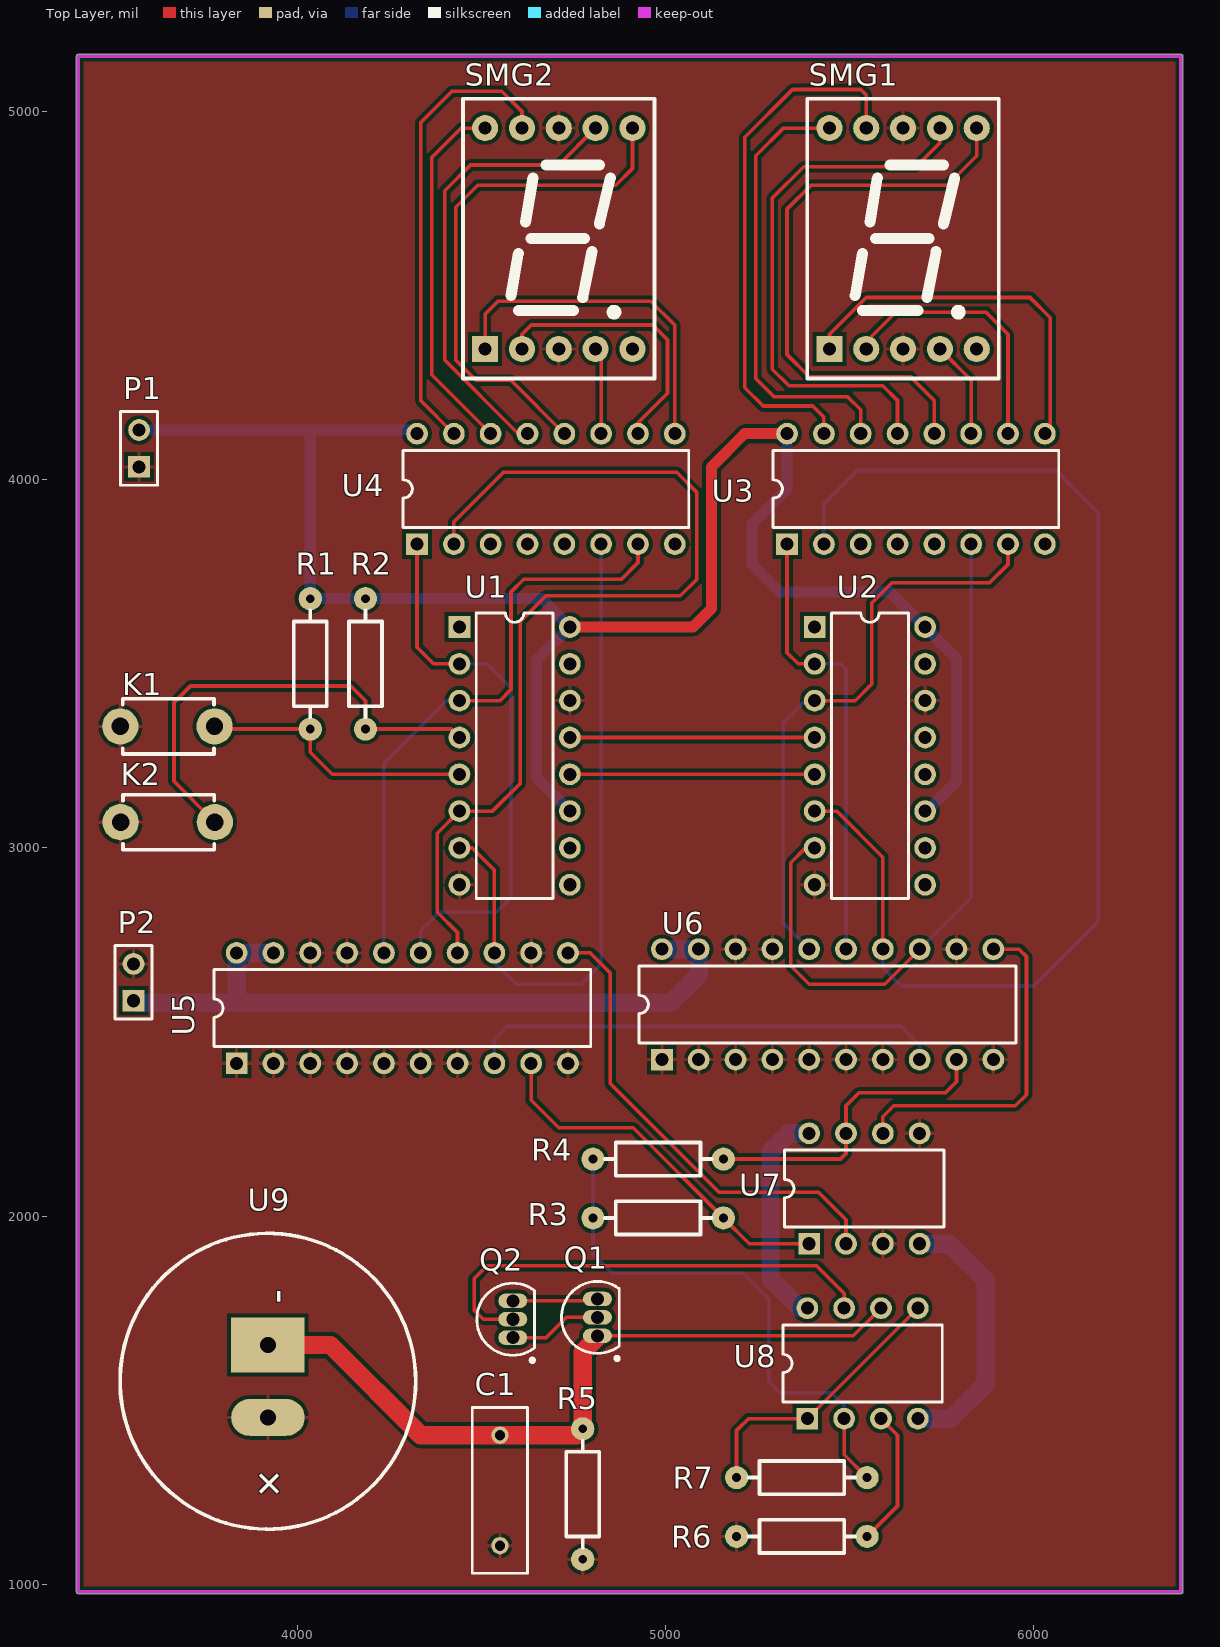
[diagram p0: Top Layer view]
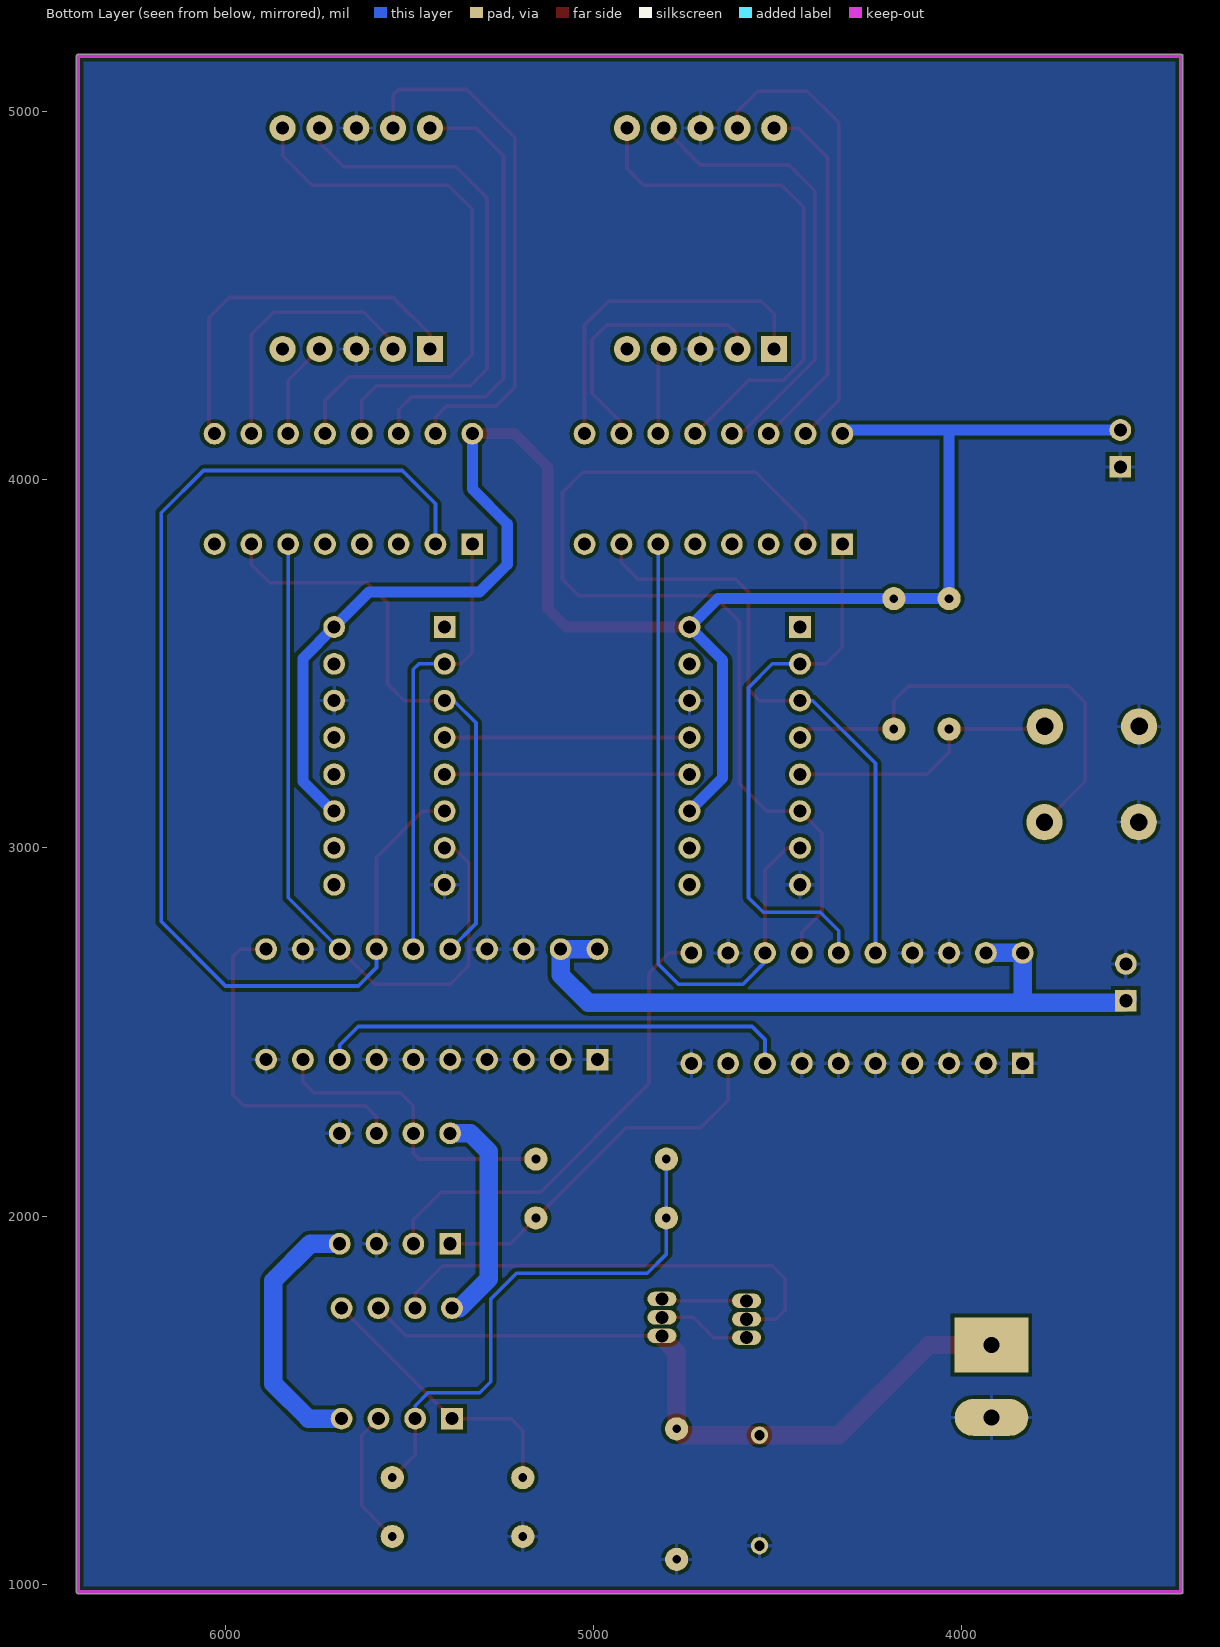
[diagram p1: Bottom Layer view, seen from below]
# Altium PCB MISC84311.PcbDoc
Units mil, origin at the board's own origin, x right, y up, seen from the top; angles counter-clockwise.
Board outline 3005.03 x 4180.03 mil, 2 copper layers (Top Layer, Bottom Layer); 25 components, 43 nets, 172 pads, 0 vias.

## Layer stack, top to bottom (the 12.6 mil dielectric is the usual default, probably not edited)
Top Solder: solder mask 0.4, Solder Resist, Dk 3.5
Top Layer: signal copper 1.4
Dielectric 1: dielectric 12.6, FR-4, Dk 4.8
Bottom Layer: signal copper 1.4
Bottom Solder: solder mask 0.4, Solder Resist, Dk 3.5

## Board outline
3399.99,980 ccw(c3405,980) 3405,974.99 6400,974.99 ccw(c6400,980) 6405.02,980 6405.02,5150 ccw(c6400,5150) 6400,5155.02 3405,5155.02 ccw(c3405,5150) 3399.99,5150

## Design rules (kind name [scope] priority, off if disabled: settings)
Clearance [All] p1: gap=10
HoleSize [All] p1: absolutevalues=TRUE maxlimit=99999 minlimit=1 maxpercent=80.000 minpercent=20.000
MinimumSolderMaskSliver [All] p1: minsoldermaskwidth=0
PolygonConnect [All] p1: connectstyle=Relief reliefconductorwidth=10 reliefentries=4 polygonreliefangle="90 Angle" airgapwidth=10
RoutingVias [All] p1: holewidth=28 width=50 viastyle="Through Hole" minholewidth=28 minwidth=50 maxholewidth=28 maxwidth=50
SilkToSilkClearance [All] p1: silktosilkclearance=0
SilkToSolderMaskClearance [IsPad] p1: minsilkscreentomaskgap=0 clearancetoexposedcopper=TRUE
SolderMaskExpansion [All] p1: expansion=4
Width [All] p1: maxlimit=50 minlimit=10 preferedwidth=10
26 further rules are at their usual default settings.

## Components (designator, comment, footprint, x,y, rotation, side; value= is the part's Value field where it differs from the comment)
C1 "100UF" RAD-0.3 4550,1255 r90 top
K1 "KEY" DIP-3X6X4.3 3519.09,3330 r0 top
K2 "KEY" DIP-3X6X4.3 3520,3070 r0 top
P1 "Header 2" HDR1X2 3570,4035 r90 top
P2 "Header 2" HDR1X2 3555,2585 r90 top
Q1 "2N3055" TO-92A 4815,1725 r0 top
Q2 "2N3904" TO-92A 4585,1720 r0 top
R1 "10K" "RS 1/4W" 4035,3500 r90 top
R2 "10K" "RS 1/4W" 4185,3500 r90 top
R3 "100K" "RS 1/4W" 4980,1995 r0 top
R4 "10K" "RS 1/4W" 4980,2155 r0 top
R5 "10K" "RS 1/4W" 4775,1245 r270 top
R6 "10K" "RS 1/4W" 5370,1130 r0 top
R7 "10K" "RS 1/4W" 5370,1290 r180 top
SMG1 "5011A" "SMG 0.5-1P" 5645,4655 r0 top
SMG2 "5011A" "SMG 0.5-1P" 4710,4655 r0 top
U1 "SN74LS192N" 648-08 4590,3250 r270 top
U2 "SN74LS192N" 648-08 5555,3250 r270 top
U3 "SN74LS48N" N016D 5680,3975 r0 top
U4 "SN74LS48N" N016D 4675,3975 r0 top
U5 "DAC0832" J20A 4285,2565 r0 top
U6 "DAC0832" J20A 5440,2575 r0 top
U7 "NE5532" P008 5540,2075 r0 top
U8 "NE5532" P008 5535,1600 r0 top
U9 "Volts" "CAPACITANCE 1 FARAD 5,5 VOLT" 3920,1551.58 r90 top

## Footprints (in the part's own frame and the unit in brackets; to place one, negate y for a bottom-side part, rotate by r counter-clockwise, add the part's x,y. Pads: shape width x height; smd on the part's side, far side on the other; paste and mask are expansions set on the pad)
648-08 [mm] "DIP; 16 Leads; Row Spacing 7.62 mm; Pitch 2.54 mm"
  rect 1.5x1.5 hole 0.9: 1(-8.89,-3.81)
  round 1.5 hole 0.9: 2(-6.35,-3.81) 3(-3.81,-3.81) 4(-1.27,-3.81) 5(1.27,-3.81) 6(3.81,-3.81) 7(6.35,-3.81) 8(8.89,-3.81) 9(8.89,3.81) 10(6.35,3.81) 11(3.81,3.81) 12(1.27,3.81) 13(-1.27,3.81) 14(-3.81,3.81) 15(-6.35,3.81) 16(-8.89,3.81)
  silkscreen extent -9.85,-2.65 9.85,2.65
"CAPACITANCE 1 FARAD 5,5 VOLT" [mil]
  rect 150x200 hole 43.31 paste+0 mask+2: 1(98.42,0)
  oval 100x200 hole 43.31 paste+0 mask+2: 2(-98.4,0)
  silkscreen extent -402,-402 402,401
DIP-3X6X4.3 [mm]
  round 2.5 hole 1.2: 1(0,0) 3(6.5,0)
  silkscreen extent 0.16,-1.9 6.46,1.9, body extent -0.64,-1.75 7.19,1.75, height 4.31
HDR1X2 [mm] "Connector; Header; 2 Position"
  rect 1.5x1.5 hole 0.9: 1(0,0)
  round 1.5 hole 0.9: 2(2.54,0)
  silkscreen extent -1.27,-1.27 3.81,1.27
J20A [mm] "DIP; 20 Leads; Row Spacing 7.62 mm; Pitch 2.54 mm"
  rect 1.5x1.5 hole 0.9: 1(-11.43,-3.81)
  round 1.5 hole 0.9: 2(-8.89,-3.81) 3(-6.35,-3.81) 4(-3.81,-3.81) 5(-1.27,-3.81) 6(1.27,-3.81) 7(3.81,-3.81) 8(6.35,-3.81) 9(8.89,-3.81) 10(11.43,-3.81) 11(11.43,3.81) 12(8.89,3.81) 13(6.35,3.81) 14(3.81,3.81) 15(1.27,3.81) 16(-1.27,3.81) 17(-3.81,3.81) 18(-6.35,3.81) 19(-8.89,3.81) 20(-11.43,3.81)
  silkscreen extent -13,-2.65 13,2.65
N016D [mm] "DIP; 16 Leads; Row Spacing 7.62 mm; Pitch 2.54 mm"
  rect 1.5x1.5 hole 0.9: 1(-8.89,-3.81)
  round 1.5 hole 0.9: 2(-6.35,-3.81) 3(-3.81,-3.81) 4(-1.27,-3.81) 5(1.27,-3.81) 6(3.81,-3.81) 7(6.35,-3.81) 8(8.89,-3.81) 9(8.89,3.81) 10(6.35,3.81) 11(3.81,3.81) 12(1.27,3.81) 13(-1.27,3.81) 14(-3.81,3.81) 15(-6.35,3.81) 16(-8.89,3.81)
  silkscreen extent -9.85,-2.65 9.85,2.65
P008 [mm] "DIP; 8 Leads; Row Spacing 7.62 mm; Pitch 2.54 mm"
  rect 1.5x1.5 hole 0.9: 1(-3.81,-3.81)
  round 1.5 hole 0.9: 2(-1.27,-3.81) 3(1.27,-3.81) 4(3.81,-3.81) 5(3.81,3.81) 6(1.27,3.81) 7(-1.27,3.81) 8(-3.81,3.81)
  silkscreen extent -5.5,-2.65 5.5,2.65
RAD-0.3 [mm] "Radial Cap, Thru-Hole; 2 Leads; 0.3 in Pin Spacing"
  round 1.2 hole 0.7: 1(-3.81,0) 2(3.81,0)
  silkscreen extent -5.71,-1.91 5.71,1.91
"RS 1/4W" [mm] "直插色环电阻，脚距9mm，直径2.3mm"
  round 1.6 hole 0.6: 1(-4.5,0) 2(4.5,0)
  silkscreen extent -3.68,-1.14 3.68,1.14, body extent -4.72,-1.16 4.73,1.16, height 2.32
"SMG 0.5-1P" [mm] "12.7*19*8mm(长宽厚)"
  rect 1.8x1.8 hole 0.9: 1(-5.08,-7.62)
  round 1.8 hole 0.9: 2(-2.54,-7.62) 3(0,-7.62) 4(2.54,-7.62) 5(5.08,-7.62) 6(5.08,7.62) 7(2.54,7.62) 8(0,7.62) 9(-2.54,7.62) 10(-5.08,7.62)
  silkscreen extent -6.6,-9.65 6.6,9.65, body extent -6.35,-9.5 6.35,9.5, height 8
TO-92A [mm] "TO, Flat Index; 3 In-Line, Axial Leads; Body Dia. 4.5mm; Leads 0.51 x 0.48 mm (max)"
  oval 2x1 hole 0.9: 1(0,-1.27) 2(0,0) 3(0,1.27)
  silkscreen extent -2.48,-2.95 1.5,2.48, body extent -2.48,-2.5 1.5,2.5, height 6.86

## Part data
C1: library part Cap, "Capacitor"
P1 P2: "Header, 2-Pin"
Q1: library part 2N3904, "NPN General Purpose Amplifier"
Q2: "NPN General Purpose Amplifier"
R1 R2 R3 R4 R5 R6 R7: library part R-S, "Color-band resistor"
SMG1 SMG2: "0.5-inch 1-digit common-cathode seven-segment display"
U1 U2: "Presettable BCD Decade Up/Down Counter"
U3 U4: "BCD-to-Seven-Segment Decoder/Driver"
U5 U6: library part DAC0832LCJ, "8-Bit uP-Compatible, Double-Buffered Digital-to-Analog Converter"
U7 U8: library part NE5532AP, "Dual Low-Noise Operational Amplifier"

## Nets (pads, with @x,y where several pads share a name; then routed paths per layer and width w, separated by ;. In a path a pad name is that pad's centre, name@x,y a point inside that pad or via, vN(x,y) a via of type N, cw(c..) or ccw(c..) an arc to the next point about the centre after c; other vN are vias at no path point)
+5V: P1.2 R1.2 R2.2 U1.11 U1.16 U2.11 U2.16 U3.16 U4.16 | length 5071.7
  Top Layer w30: U1.16 5075,3600 5125,3650 5125,4035 5215,4125 U3.16
  Bottom Layer w30: P1.2 4030,4135 ; U4.16 4315,4135 4030,4135 ; U1.11 4650,3190 4650,3510 U1.16 4662.83,3677.17 R2.2 R1.2 4035,4130 4030,4135 ; U3.16 5330,3975 5235,3880 5235,3770 5310,3695 5610,3695 U2.16 5790,3515 5790,3180 5710,3100 U2.11
+12V: P2.1 U5.19 U5.20 U6.19 U6.20 | length 1980.2
  Bottom Layer w50: P2.1@3550,2590 P2.1 3560,2580 3835,2580 ; U5.19 U5.20 3835,2580 ; U6.20 U6.19 5090,2655 5015,2580 3835,2580
+15V: U7.8 U8.8 | length 603.8
  Bottom Layer w50: U8.8 5365,1750 5285,1830 5285,2175 5335,2225 U7.8
-15V: U7.4 U8.4 | length 725.8
  Bottom Layer w50: U8.4 5775,1450 5870,1545 5870,1825 5770,1925 U7.4
GND: C1.1 K1.1 K2.1 P1.1 P2.2 R5.2 R6.1 SMG1.3 SMG1.8 SMG2.3 SMG2.8 U1.8 U1.14 U2.8 U2.14 U5.1 U5.2 U5.3 U5.4 U5.5 U5.6 U5.7 U5.10 U5.12 U5.17 U5.18 U6.1 U6.2 U6.3 U6.4 U6.5 U6.6 U6.7 U6.10 U6.12 U6.17 U6.18 U7.3 U7.5 U9.2
NetC1_2: C1.2 Q1.1 R5.1 U8.6 U9.1 | length 2032.7
  Top Layer w10: Q1.1@4812.66,1672.66 Q1.1 5510,1675 U8.6
  Top Layer w50: U9.1 4090,1650 4335,1405 C1.2 4757.83,1405 R5.1 4775,1630.32 Q1.1@4815,1670.32
NetK1_3: K1.3 R1.1 U1.5 | length 755.7
  Top Layer w10: K1.3 3782.17,3322.83 R1.1 4035,3260 4095,3200 U1.5
NetK2_3: K2.3 R2.1 U1.4 | length 1267.8
  Top Layer w10: K2.3 3665,3180.91 3665,3395 3710,3440 4145,3440 4185,3400 R2.1 4417.17,3322.83 U1.4
NetQ1_2: Q1.2 Q2.1 | length 252.8
  Top Layer w10: Q2.1 4675,1670 4730,1725 Q1.2
NetQ1_3: Q1.3 Q2.3 | length 232.1
  Top Layer w10: Q2.3 4810,1770 Q1.3
NetQ2_2: Q2.2 U8.7 | length 1290.9
  Top Layer w10: Q2.2 4505,1720 4480,1745 4480,1830 4515,1865 5410,1865 5485,1790 U8.7
NetR3_1: R3.1 R4.1 R7.1 U8.2 | length 1463.3
  Top Layer w10: U8.2 5485,1352.17 R7.1
  Bottom Layer w10: R4.1 R3.1 4802.83,1897.17 4855,1845 5210,1845 5280,1775 5280,1550 5310,1520 5450,1520 5485,1485 U8.2
NetR3_2: R3.2 U5.9 U7.1 | length 1016.5
  Top Layer w10: U5.9 4635,2315 4710,2240 4912.17,2240 R3.2 5227.17,1925 U7.1
NetR4_2: R4.2 U6.9 U7.7 | length 856
  Top Layer w10: R4.2 5475,2155 5490,2170 U7.7 5490,2300 5525,2335 5760,2335 5790,2365 U6.9
NetR6_2: R6.2 U8.3 | length 373
  Top Layer w10: R6.2 5630,1212.83 5630,1405 U8.3
NetR7_2: R7.2 U8.1 U8.5 | length 757.6
  Top Layer w10: R7.2 5192.83,1417.83 5225,1450 U8.1 U8.5
NetSMG1_1: SMG1.1 U3.9 | length 1025.4
  Top Layer w10: SMG1.1 5445,4395 5545,4495 5990,4495 6045,4440 6045,4140 U3.9
NetSMG1_2: SMG1.2 U3.10 | length 733
  Top Layer w10: SMG1.2 5545,4375 5625,4455 5870,4455 5930,4395 U3.10
NetSMG1_4: SMG1.4 U3.11 | length 265.2
  Top Layer w10: SMG1.4 5830,4270 U3.11
NetSMG1_6: SMG1.6 U3.12 | length 1586.8
  Top Layer w10: U3.12 5730,4215 5665,4280 5390,4280 5330,4340 5330,4735 5395,4800 5765,4800 5845,4880 SMG1.6
NetSMG1_7: SMG1.7 U3.13 | length 1487.3
  Top Layer w10: U3.13 5630,4215 5590,4255 5335,4255 5290,4300 5290,4765 5375,4850 5680,4850 5745,4915 SMG1.7
NetSMG1_9: SMG1.9 U3.15 | length 1453.2
  Top Layer w10: U3.15 5430,4170 5400,4200 5265,4200 5215,4250 5215,4930 5345,5060 5530,5060 5545,5045 SMG1.9
NetSMG1_10: SMG1.10 U3.14 | length 1221.3
  Top Layer w10: SMG1.10 5320,4955 5245,4880 5245,4275 5295,4225 5495,4225 5530,4190 U3.14
NetSMG2_1: SMG2.1 U4.9 | length 946.4
  Top Layer w10: SMG2.1 4510,4450 4545,4485 4960,4485 5025,4420 U4.9
NetSMG2_2: SMG2.2 U4.10 | length 750.1
  Top Layer w10: SMG2.2 4610,4395 4635,4420 4965,4420 5005,4380 5005,4235 4925,4155 U4.10
NetSMG2_4: SMG2.4 U4.11 | length 236.2
  Top Layer w10: SMG2.4 4825,4340 U4.11
NetSMG2_6: SMG2.6 U4.12 | length 1426.3
  Top Layer w10: U4.12 4580,4270 4485,4270 4430,4325 4430,4740 4490,4800 4865,4800 4910,4845 SMG2.6
NetSMG2_7: SMG2.7 U4.13 | length 1248.3
  Top Layer w10: U4.13 4600,4125 4400,4325 4400,4785 4470,4855 4710,4855 SMG2.7
NetSMG2_9: SMG2.9 U4.15 | length 1260.3
  Top Layer w10: U4.15 4335,4215 4335,4970 4420,5055 4555,5055 4610,5000 SMG2.9
NetSMG2_10: SMG2.10 U4.14 | length 994.4
  Top Layer w10: SMG2.10 4445,4955 4365,4875 4365,4285 U4.14
NetU1_2: U1.2 U4.1 U5.15 | length 1492.8
  Top Layer w10: U4.1 4325,3545 4370,3500 U1.2
  Bottom Layer w10: U5.15 4335,2775 4385,2825 4540,2825 4580,2865 4580,3435 4515,3500 U1.2
NetU1_3: U1.3 U4.7 U5.16 | length 1636
  Top Layer w10: U1.3 4550,3400 4580,3430 4580,3695 4615,3730 4880,3730 4925,3775 U4.7
  Bottom Layer w10: U5.16 4235,3230 4405,3400 U1.3
NetU1_6: U1.6 U4.2 U5.14 | length 2630
  Top Layer w10: U4.2 4425,3885 4560,4020 5030,4020 5085,3965 5085,3730 5040,3685 4675,3685 4605,3615 4605,3175 4530,3100 U1.6 4380,3040 4380,2825 4435,2770 U5.14
NetU1_7: U1.7 U4.6 U5.13 | length 1847.5
  Top Layer w10: U1.7 4475,3000 4535,2940 U5.13
  Bottom Layer w10: U5.13 4535,2690 4595,2630 4770,2630 4825,2685 U4.6
NetU1_12: U1.12 U2.5 | length 665
  Top Layer w10: U1.12 U2.5
NetU1_13: U1.13 U2.4 | length 665
  Top Layer w10: U1.13 U2.4
NetU2_2: U2.2 U3.1 U6.15 | length 1233.6
  Top Layer w10: U3.1 5330,3530 5360,3500 U2.2
  Bottom Layer w10: U2.2 5475,3500 5490,3485 U6.15
NetU2_3: U2.3 U3.7 U6.16 | length 1616
  Top Layer w10: U2.3 5515,3400 5560,3445 5560,3665 5615,3720 5880,3720 5930,3770 U3.7
  Bottom Layer w10: U6.16 5320,2795 5320,3340 5380,3400 U2.3
NetU2_6: U2.6 U3.2 U6.14 | length 3264.9
  Top Layer w10: U2.6 5465,3100 5590,2975 U6.14
  Bottom Layer w10: U3.2 5430,3935 5520,4025 6060,4025 6175,3910 6175,2800 6000,2625 5640,2625 5590,2675 U6.14
NetU2_7: U2.7 U3.6 U6.13 | length 1929.6
  Top Layer w10: U2.7 5380,3000 5340,2960 5340,2680 5390,2630 5595,2630 U6.13
  Bottom Layer w10: U6.13 5830,2865 U3.6
NetU5_8: U5.8 U6.8 | length 1295.2
  Bottom Layer w10: U5.8 4535,2480 4570,2515 5640,2515 5690,2465 U6.8
NetU5_11: U5.11 U7.2 | length 1296
  Top Layer w10: U5.11 4795,2715 4850,2660 4850,2360 5145,2065 5415,2065 5490,1990 U7.2
NetU6_11: U6.11 U7.6 | length 933.1
  Top Layer w10: U7.6 5590,2270 5620,2300 5950,2300 5980,2330 5980,2705 5960,2725 U6.11
pads on no net: SMG1.5 SMG2.5 U1.1 U1.9 U1.10 U1.15 U2.1 U2.9 U2.10 U2.12 U2.13 U2.15 U3.3 U3.4 U3.5 U3.8 U4.3 U4.4 U4.5 U4.8

## Polygon pours and split planes (outlines as drawn)
GND on Bottom Layer "D" (solid, remove dead copper, pour order 0): 2445,5425 7280,5425 7280,860 6980,560 6675,865 2245,865
GND on Top Layer "D" (solid, remove dead copper, pour order 2): 2700,5595 6455,5595 6460,5590 6710,5340 6710,1380 6710,895 6290,475 6195,570 2840,570

## Keep-outs
Keep-Out Layer:
  lines w10: 3405,5015 3405,5150 6400,5150 6400,980 3765,980 3405,980 3405,5025